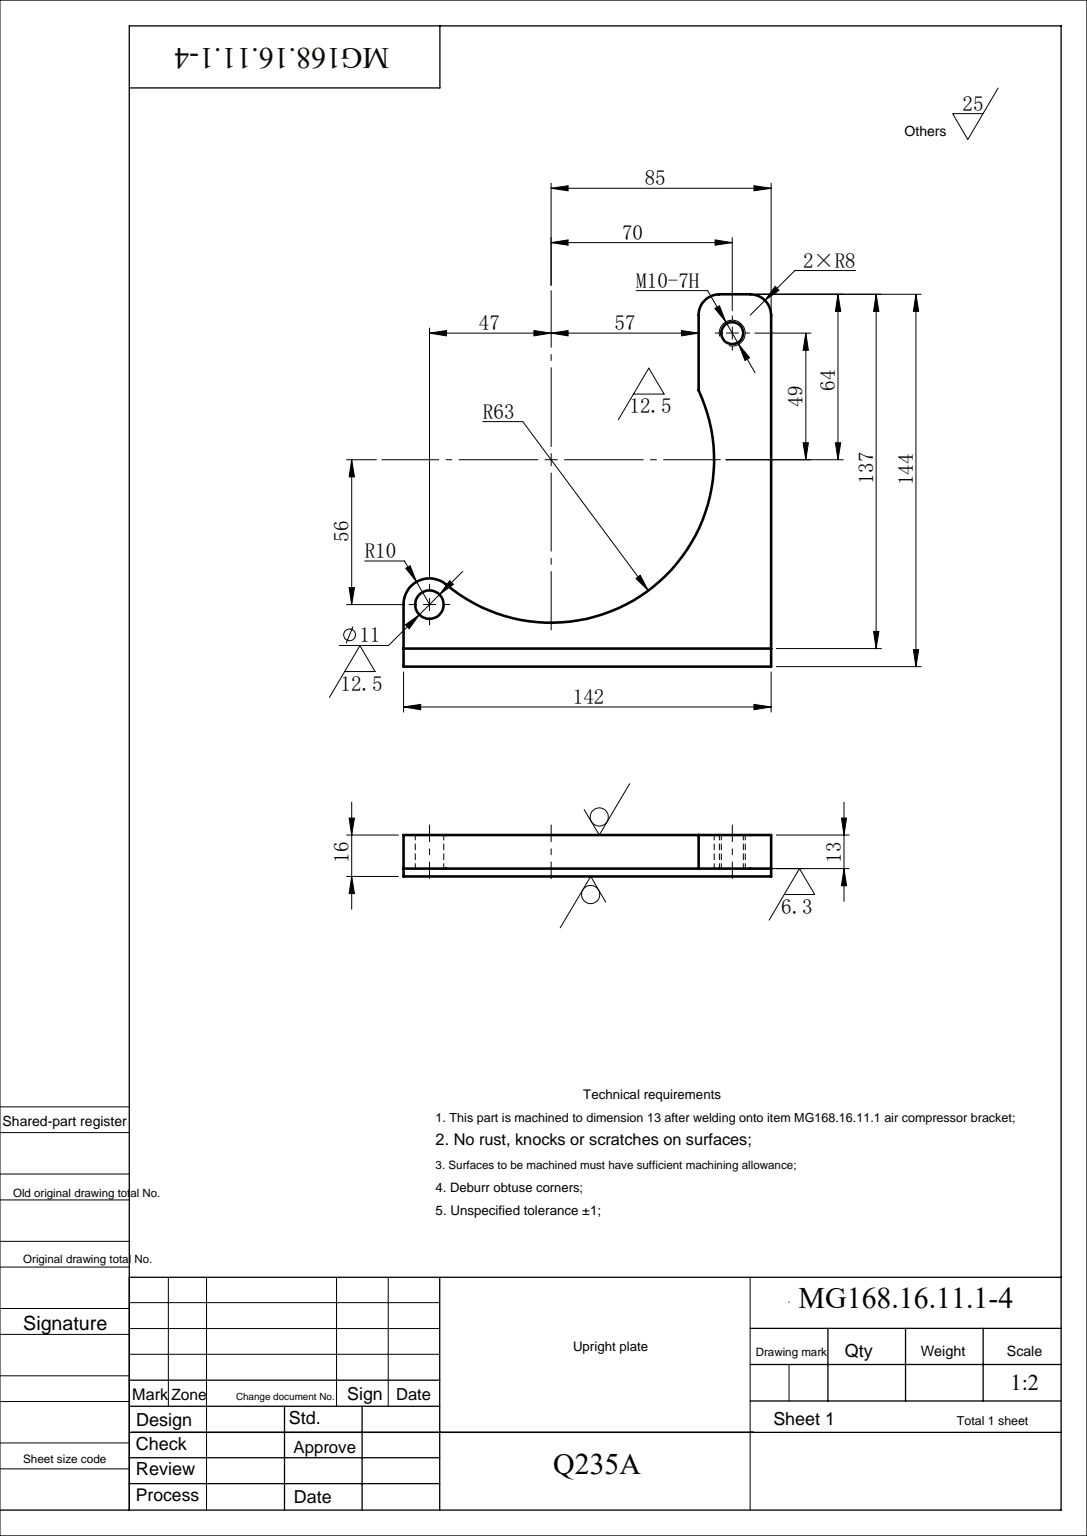
SolidWorks part; units mm, degrees
material "Q235A"
ref_plane "Front Plane" through (0, 0, 0) normal (0, 0, 1) x (1, 0, 0)
ref_plane "Top Plane" through (0, 0, 0) normal (0, 1, 0) x (1, 0, 0)
ref_plane "Right Plane" through (0, 0, 0) normal (1, 0, 0) x (0, 0, -1)
sketch "Sketch1" plane through (0, 0, 0) normal (0, 0, 1) x (1, 0, 0)
  line L0 (28, 144) -> (28, 106.8328)
  line L1 (0, 0) -> (142, 0)
  line L2 (0, 0) -> (0, 144)
  line L3 (0, 144) -> (28, 144)
  line L4 (142, 0) -> (142, 24.143)
  arc A0 (28, 106.8328) -> (125.5616, 31.7947) centre (85, 80) ccw
  circle A1 centre (132, 24) radius 5.5
  arc A2 (142, 24.143) -> (125.5616, 31.7947) centre (132, 24.143) ccw
  dimension "D1" = 63
  dimension "D5" = 11
  dimension "D10" = 10
  dimension "D2" = 144
  dimension "D3" = 142
  dimension "D4" = 28
  dimension "D6" = 24
  dimension "D7" = 56
  dimension "D8" = 10
  dimension "D9" = 47
extrude "Boss-Extrude1" add sketch "Sketch1" along normal mid plane 13
sketch "Sketch2" plane through (0, 0, -6.5) normal (0, 0, 1) x (1, 0, 0)
  line L0 (142, 0) -> (142, 24.143) construction
  line L1 (0, 0) -> (142, 0)
  line L2 (0, 0) -> (0, 7)
  line L3 (0, 7) -> (142, 7)
  line L4 (142, 0) -> (142, 7)
  dimension "D1" = 7
extrude "Boss-Extrude2" add sketch "Sketch2" against normal blind 3
hole_wizard "M10 Tapped Hole1" positions "Sketch4" profile "Sketch3" tap size "M10" standard "GB" end condition through all
sketch "Sketch4" plane through (0, 0, 6.5) normal (0, 0, 1) x (1, 0, 0)
  circle A0 centre (132, 24) radius 5.5 construction
  point P0 (15, 129)
  dimension "D1" = 105
  dimension "D2" = 117
sketch "Sketch3" plane through (15, 129, 6.5) normal (1, 0, 0) x (0, -1, 0)
  line L0 (0, 0) -> (0, 16)
  line L1 (0, 16) -> (4.25, 16)
  line L2 (4.25, 16) -> (4.25, 0)
  line L5 (4.25, 0) -> (0, 0)
  line L11 (0, -6.35) -> (0, 107.95) construction
  dimension "通孔螺纹孔钻头直径" = 8.5
  dimension "通孔螺纹孔钻头深度" = 16
cosmetic thread "Hole Thread1" parameters "D2"=10
fillet "Fillet1" radius 8 2 edges at (0, 144, 0) (28, 144, 0)
